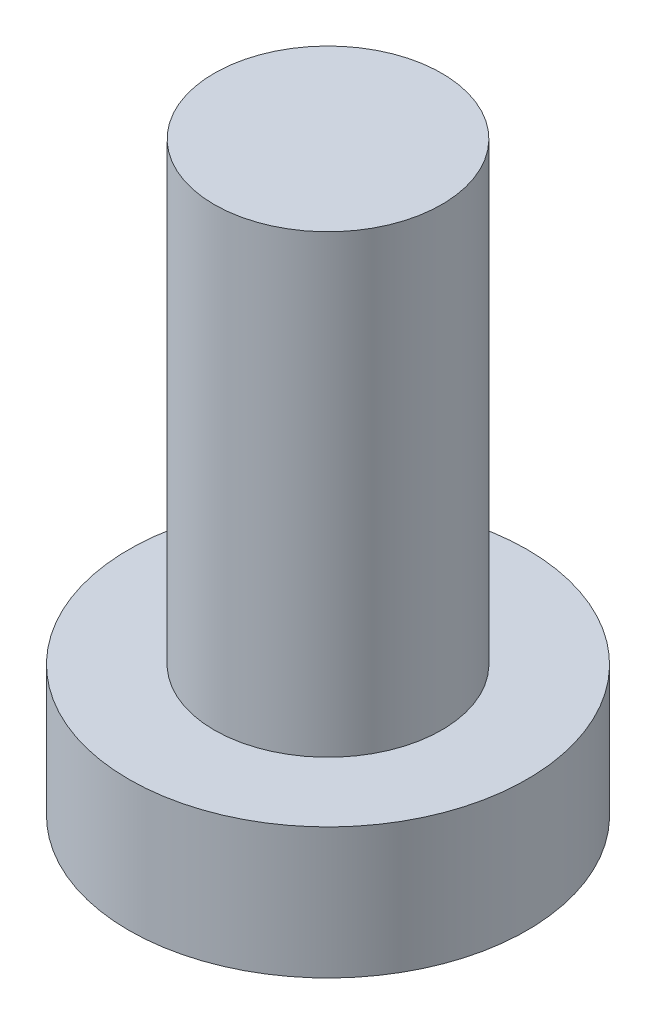
SolidWorks part; units mm, degrees
ref_plane "前视基准面" through (0, 0, 0) normal (0, 0, 1) x (1, 0, 0)
ref_plane "上视基准面" through (0, 0, 0) normal (0, 1, 0) x (1, 0, 0)
ref_plane "右视基准面" through (0, 0, 0) normal (1, 0, 0) x (0, 0, -1)
sketch "草图1" plane through (0, 0, 0) normal (0, 1, 0) x (1, 0, 0)
  circle A0 centre (0, 0) radius 2
  dimension "D1" = 4
extrude "凸台-拉伸1" add sketch "草图1" along normal blind 8
sketch "草图2" plane through (0, 0, 0) normal (0, -1, 0) x (1, 0, 0)
  circle A0 centre (0, 0) radius 3.5
  dimension "D1" = 7
extrude "凸台-拉伸2" add sketch "草图2" along normal blind 2.3
